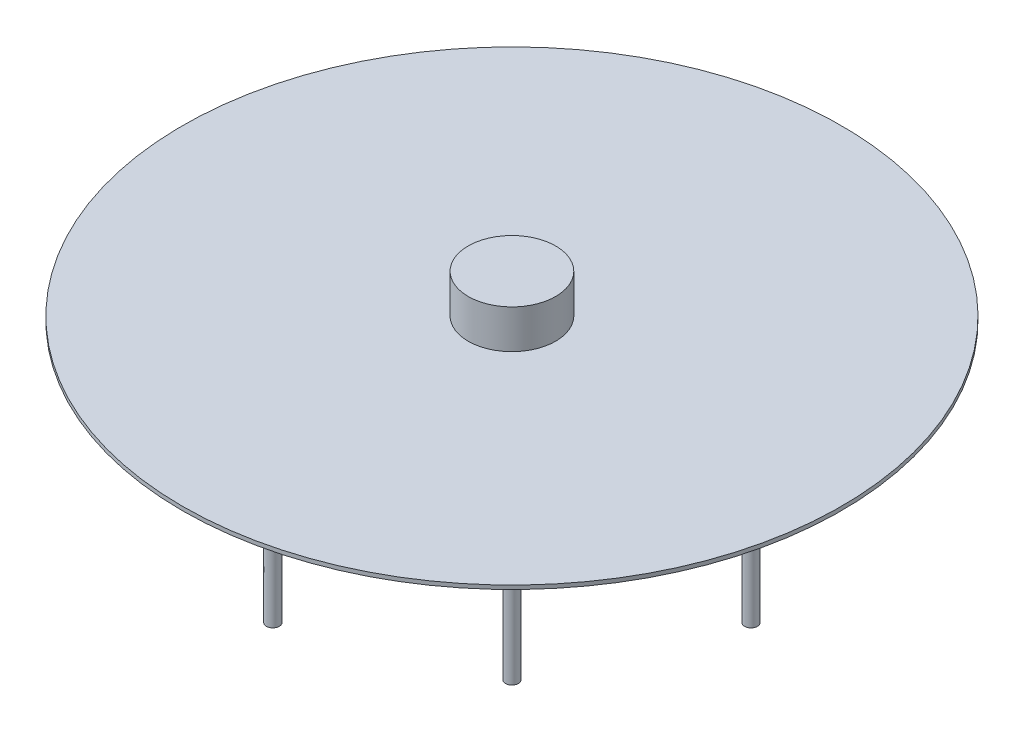
from build123d import *

# Parameters (mm, degrees)
SKETCH1_R           = 225
BOSS_EXTRUDE2_DEPTH = 10
SKETCH2_R           = 5
BOSS_EXTRUDE3_DEPTH = 100
SKETCH3_R           = 255
BOSS_EXTRUDE5_DEPTH = 3
SKETCH7_R           = 33.849496271
BOSS_EXTRUDE6_DEPTH = 30


with BuildPart() as part:
    # Sketch1 → Boss-Extrude2 (new body)
    with BuildSketch(Plane(origin=(0, 0, 0), x_dir=(1, 0, 0), z_dir=(0, 1, 0))):
        with Locations(Location((0, 0, 0), (0, 0, 270))):
            Circle(SKETCH1_R)
    extrude(amount=BOSS_EXTRUDE2_DEPTH)

    # Sketch2 → Boss-Extrude3 (add)
    with BuildSketch(Plane.XZ):
        with Locations(Location((-185, 0, 0), (0, 0, 90))):
            Circle(SKETCH2_R)
        with Locations(Location((-130.81475452, 130.81475452, 0), (0, 0, 90))):
            Circle(SKETCH2_R)
        with Locations(Location((0, 185, 0), (0, 0, 90))):
            Circle(SKETCH2_R)
        with Locations(Location((130.81475452, 130.81475452, 0), (0, 0, 90))):
            Circle(SKETCH2_R)
        with Locations(Location((185, 0, 0), (0, 0, 90))):
            Circle(SKETCH2_R)
        with Locations(Location((130.81475452, -130.81475452, 0), (0, 0, 90))):
            Circle(SKETCH2_R)
        with Locations(Location((0, -185, 0), (0, 0, 90))):
            Circle(SKETCH2_R)
        with Locations(Location((-130.81475452, -130.81475452, 0), (0, 0, 90))):
            Circle(SKETCH2_R)
    extrude(amount=BOSS_EXTRUDE3_DEPTH)

    # Sketch3 → Boss-Extrude5 (add)
    with BuildSketch(Plane(origin=(0, 10, 0), x_dir=(1, 0, 0), z_dir=(0, 1, 0))):
        with Locations(Location((0, 0, 0), (0, 0, 270))):
            Circle(SKETCH3_R)
    extrude(amount=BOSS_EXTRUDE5_DEPTH)

    # Sketch7 → Boss-Extrude6 (add)
    with BuildSketch(Plane(origin=(0, 13, 0), x_dir=(1, 0, 0), z_dir=(0, 1, 0))):
        with Locations(Location((0, 0, 0), (0, 0, 270))):
            Circle(SKETCH7_R)
    extrude(amount=BOSS_EXTRUDE6_DEPTH)


solid = part.part
